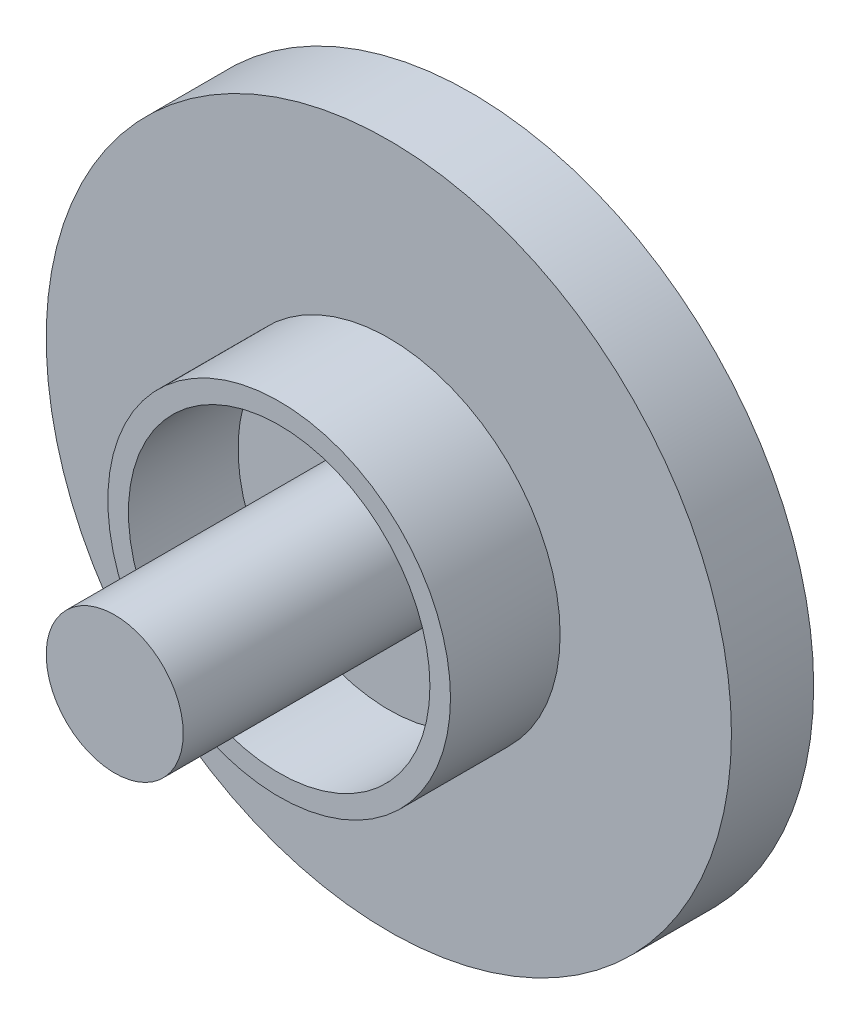
SolidWorks part; units mm, degrees
ref_plane "前视基准面" through (0, 0, 0) normal (0, 0, 1) x (1, 0, 0)
ref_plane "上视基准面" through (0, 0, 0) normal (0, 1, 0) x (1, 0, 0)
ref_plane "右视基准面" through (0, 0, 0) normal (1, 0, 0) x (0, 0, -1)
other "Configuration Table"
sketch "草图1" plane through (0, 0, 0) normal (0, 0, 1) x (1, 0, 0)
  circle A0 centre (0, 0) radius 25
extrude "凸台-拉伸1" add sketch "草图1" along normal blind 6
sketch "草图2" plane through (0, 0, 6) normal (0, 0, 1) x (1, 0, 0)
  circle A0 centre (0, 0) radius 11
  circle A1 centre (0, 0) radius 12.5
extrude "凸台-拉伸2" add sketch "草图2" along normal blind 8
sketch "草图3" plane through (0, 0, 6) normal (0, 0, 1) x (1, 0, 0)
  circle A0 centre (0, 0) radius 5
extrude "凸台-拉伸3" add sketch "草图3" along normal blind 20
sketch "草图5" plane through (0, 0, 0) normal (0, 0, -1) x (-1, 0, 0)
  circle A0 centre (0, 0) radius 10.475
  circle A1 centre (0, 0) radius 11.5
extrude "凸台-拉伸4" add sketch "草图5" along normal blind 4
sketch "草图6" plane through (0, 0, 0) normal (0, 0, -1) x (-1, 0, 0)
  circle A0 centre (0, 0) radius 1.425
extrude "凸台-拉伸5" add sketch "草图6" along normal blind 10
